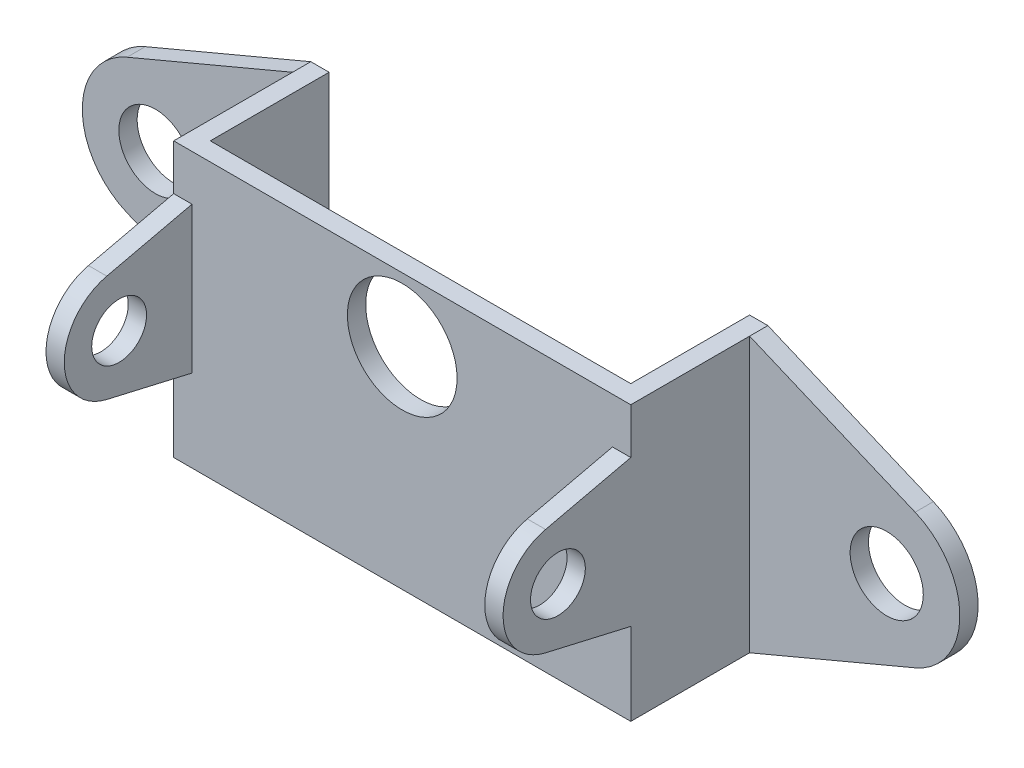
SolidWorks part; units mm, degrees
material "1.4000 (X6Cr13)"
ref_plane "Front Plane" through (0, 0, 0) normal (0, 0, 1) x (1, 0, 0)
ref_plane "Top Plane" through (0, 0, 0) normal (0, 1, 0) x (1, 0, 0)
ref_plane "Right Plane" through (0, 0, 0) normal (1, 0, 0) x (0, 0, -1)
sketch "Sketch1" plane through (0, 0, 0) normal (0, 0, 1) x (1, 0, 0)
  line L0 (-121.5312, 170.619) -> (-121.5312, 135.4631) construction
  line L2 (-101.5312, 150.119) -> (-141.5312, 150.119) construction
  line L3 (-99.9783, 146.4328) -> (-109.0312, 142.619)
  line L6 (-101.5312, 150.119) -> (-98.6769, 150.119) construction
  line L7 (-99.9783, 153.8053) -> (-109.0312, 157.619)
  line L8 (-141.5312, 150.119) -> (-144.3855, 150.119) construction
  line L9 (-143.0841, 153.8053) -> (-134.0312, 157.619)
  line L10 (-134.0312, 157.619) -> (-134.0312, 142.619)
  line L11 (-143.0841, 146.4328) -> (-134.0312, 142.619)
  line L12 (-109.0312, 157.619) -> (-109.0312, 142.619)
  arc A0 (-99.9783, 146.4328) -> (-99.9783, 153.8053) centre (-101.5312, 150.119) ccw
  circle A1 centre (-121.5312, 133.619) radius 37 construction
  circle A2 centre (-101.5312, 150.119) radius 2
  circle A3 centre (-141.5312, 150.119) radius 2
  arc A4 (-143.0841, 146.4328) -> (-143.0841, 153.8053) centre (-141.5312, 150.119) cw
  point P13 (-107.0312, 150.119)
  point P17 (-121.5312, 150.119)
  point P22 (-136.0312, 150.119)
  dimension "D1" = 8
  dimension "D4" = 4
  dimension "D2" = 25
  dimension "D3" = 15
extrude "Boss-Extrude1" add sketch "Sketch1" along normal blind 1
sketch "Sketch2" plane through (0, 0, 0) normal (0, 0, 1) x (1, 0, 0)
  line L0 (-109.0312, 157.619) -> (-109.0312, 142.619) construction
  line L1 (-110.0312, 157.619) -> (-109.0312, 157.619)
  line L2 (-110.0312, 157.619) -> (-110.0312, 142.619)
  line L3 (-110.0312, 142.619) -> (-109.0312, 142.619)
  line L4 (-109.0312, 157.619) -> (-109.0312, 142.619)
  line L5 (-121.5312, 156.119) -> (-121.5312, 184.5603) construction
  line L6 (-121.5312, 147.6189) -> (-121.5312, 168.619) construction
  line L7 (-134.0312, 157.619) -> (-134.0312, 142.619)
  line L8 (-133.0312, 142.619) -> (-134.0312, 142.619)
  line L9 (-133.0312, 157.619) -> (-133.0312, 142.619)
  line L10 (-133.0312, 157.619) -> (-134.0312, 157.619)
  circle A0 centre (-121.5312, 154.119) radius 2 construction
  dimension "D1" = 1
extrude "Boss-Extrude2" add sketch "Sketch2" along normal blind 6.5
sketch "Sketch4" plane through (0, 0, 6.5) normal (0, 0, 1) x (1, 0, 0)
  line L0 (-109.0312, 142.619) -> (-109.0312, 157.619) construction
  line L1 (-109.0312, 157.619) -> (-134.0312, 157.619)
  line L2 (-109.0312, 157.619) -> (-109.0312, 142.619)
  line L3 (-109.0312, 142.619) -> (-134.0312, 142.619)
  line L4 (-134.0312, 157.619) -> (-134.0312, 142.619)
  line L5 (-110.0312, 142.619) -> (-109.0312, 142.619) construction
  line L6 (-109.0312, 157.619) -> (-110.0312, 157.619) construction
  line L7 (-121.5312, 167.619) -> (-121.5312, 157.619) construction
  line L8 (-134.0312, 157.619) -> (-134.0312, 142.619) construction
  circle A0 centre (-121.5312, 133.619) radius 34 construction
  circle A1 centre (-121.5312, 154.119) radius 3 construction
  circle A2 centre (-121.5312, 154.119) radius 3
extrude "Boss-Extrude3" add sketch "Sketch4" along normal blind 1
ref_plane "Plane5" through (-121.5312, 0, 0) normal (-1, 0, 0) x (0, 0, -1)
sketch "Sketch6" plane through (-134.0312, 0, 0) normal (-1, 0, 0) x (0, 0, 1)
  line L0 (11.4849, 151.119) -> (5.6757, 151.119) construction
  line L1 (11.4849, 147.119) -> (5.6757, 147.119)
  line L2 (11.4849, 155.119) -> (5.6757, 155.119)
  line L3 (11.4849, 147.119) -> (14.4849, 147.119) construction
  arc A0 (11.4849, 147.119) -> (11.4849, 155.119) centre (11.4849, 151.119) ccw
  arc A1 (5.6757, 155.119) -> (5.6757, 147.119) centre (5.6757, 151.119) ccw
  circle A3 centre (11.4849, 151.119) radius 1.5 construction
  circle A4 centre (11.4849, 151.119) radius 1.5
  point P3 (8.5803, 151.119)
extrude "Boss-Extrude4" add sketch "Sketch6" against normal blind 1
sketch "Sketch7" plane through (-134.0312, 0, 0) normal (-1, 0, 0) x (0, 0, 1)
  line L0 (12.1604, 154.042) -> (7.5, 155.119)
  line L2 (7.5, 151.119) -> (14.3956, 151.119) construction
  line L3 (12.1604, 148.1961) -> (7.5, 147.119)
  line L4 (7.5, 147.119) -> (14.5359, 146.0589)
  line L5 (14.5359, 146.0589) -> (15.7159, 151.3867)
  line L6 (15.7159, 151.3867) -> (15.3404, 156.6787)
  line L7 (15.3404, 156.6787) -> (10.7099, 160.898)
  line L8 (10.7099, 160.898) -> (7.5, 155.119)
  arc A0 (12.1604, 148.1961) -> (12.1604, 154.042) centre (11.4849, 151.119) ccw
  dimension "D1" = 3
extrude "Cut-Extrude1" cut sketch "Sketch7" against normal blind 1
sketch "Sketch8" plane through (-109.0312, 0, 0) normal (1, 0, 0) x (0, 0, -1)
  line L0 (-7.5, 142.619) -> (-7.5, 157.619) construction
  line L1 (-7.5, 155.119) -> (-12.1604, 154.042) construction
  line L2 (-12.1604, 148.1961) -> (-7.5, 147.119) construction
  line L3 (-7.5, 147.119) -> (-7.5, 155.119)
  line L4 (-7.5, 155.119) -> (-12.1604, 154.042)
  line L5 (-12.1604, 148.1961) -> (-7.5, 147.119)
  circle A0 centre (-11.4849, 151.119) radius 1.5 construction
  arc A1 (-12.1604, 154.042) -> (-12.1604, 148.1961) centre (-11.4849, 151.119) ccw construction
  circle A2 centre (-11.4849, 151.119) radius 1.5
  arc A3 (-12.1604, 154.042) -> (-12.1604, 148.1961) centre (-11.4849, 151.119) ccw
extrude "Boss-Extrude5" add sketch "Sketch8" against normal blind 1
